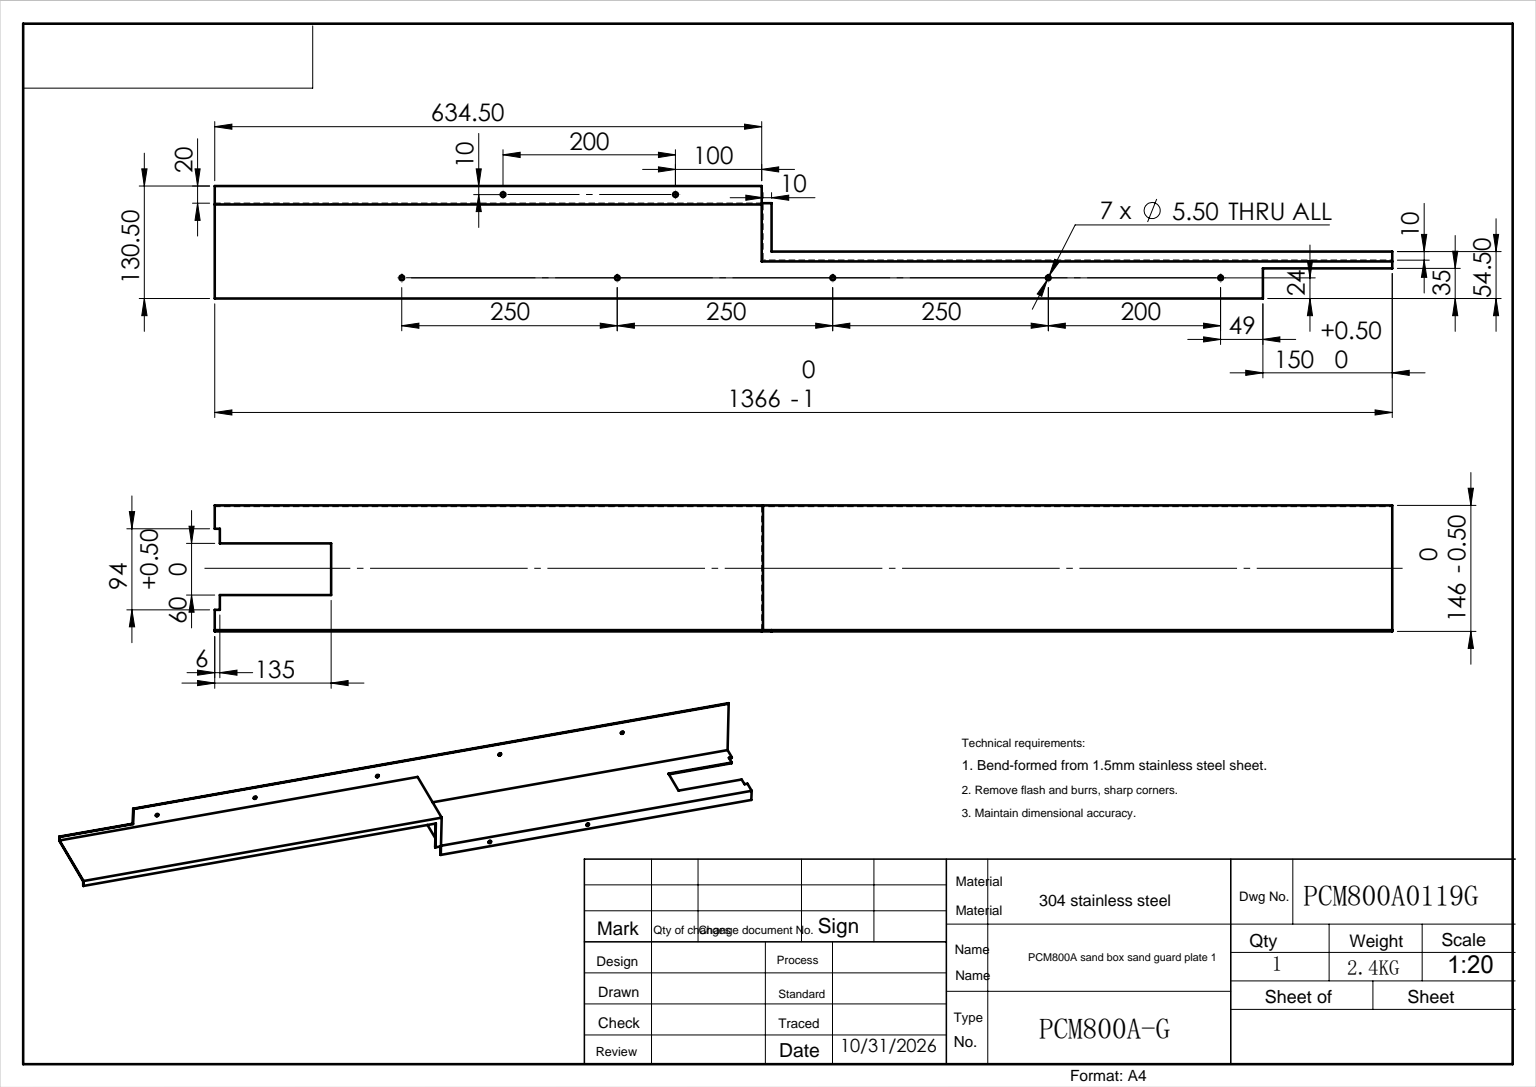
from build123d import *

# Parameters (mm, degrees)
SKETCH_1_W                  = 146
SKETCH_1_H                  = 636
EXTRUDE_1_DEPTH             = 1.5
SKETCH_2_W                  = 1.5
SKETCH_2_H                  = 636
EXTRUDE_2_DEPTH             = 109
SKETCH_4_W                  = 144.5
SKETCH_4_H                  = 1.5
EXTRUDE_4_DEPTH             = 66
EXTRUDE_5_DEPTH             = 730
SKETCH_6_W                  = 1.5
SKETCH_6_H                  = 634.5
EXTRUDE_6_DEPTH             = 20
SKETCH_7_W                  = 1.5
SKETCH_7_H                  = 730
EXTRUDE_7_DEPTH             = 10
SKETCH_8_W                  = 1.5
SKETCH_8_H                  = 56
EXTRUDE_8_DEPTH             = 10
SKETCH_10_W                 = 35
SKETCH_10_H                 = 150
CUT_EXTRUDE_2_DEPTH         = 2
HOLE_WIZARD_5_5_5_5_1_D     = 5.5
HOLE_WIZARD_5_5_5_5_2_D     = 5.5
HOLE_WIZARD_5_5_5_5_2_DEPTH = 1.5
HOLE_WIZARD_5_5_5_5_2_TIP   = 1.652366702
CUT_EXTRUDE_3_DEPTH         = 55


with BuildPart() as part:
    # 草图1 → 凸台-拉伸1 (new body)
    with BuildSketch(Plane.XY):
        with Locations((73, 318)):
            Rectangle(SKETCH_1_W, SKETCH_1_H)
    extrude(amount=EXTRUDE_1_DEPTH)

    # 草图2 → 凸台-拉伸2 (add)
    with BuildSketch(Plane.XY.offset(1.5)):
        with Locations((0.75, 318)):
            Rectangle(SKETCH_2_W, SKETCH_2_H)
    extrude(amount=EXTRUDE_2_DEPTH)

    # 草图4 → 凸台-拉伸4 (add)
    with BuildSketch(Plane.XY.offset(1.5)):
        with Locations((73.75, 0.75)):
            Rectangle(SKETCH_4_W, SKETCH_4_H)
    extrude(amount=EXTRUDE_4_DEPTH)

    # 草图5 → 凸台-拉伸5 (add)
    with BuildSketch(Plane.XZ):
        Polygon((0, 110.5), (0, 66), (146, 66), (146, 67.5), (1.5, 67.5), (1.5, 110.5), align=None)
    extrude(amount=EXTRUDE_5_DEPTH)

    # 草图6 → 凸台-拉伸6 (add)
    with BuildSketch(Plane(origin=(0, 0, 0), x_dir=(-1, 0, 0), z_dir=(0, 0, -1))):
        with Locations((-145.25, 318.75)):
            Rectangle(SKETCH_6_W, SKETCH_6_H)
    extrude(amount=EXTRUDE_6_DEPTH)

    # 草图7 → 凸台-拉伸7 (add)
    with BuildSketch(Plane(origin=(0, 0, 66), x_dir=(-1, 0, 0), z_dir=(0, 0, -1))):
        with Locations((-145.25, -365)):
            Rectangle(SKETCH_7_W, SKETCH_7_H)
    extrude(amount=EXTRUDE_7_DEPTH)

    # 草图8 → 凸台-拉伸8 (add)
    with BuildSketch(Plane.XZ):
        with Locations((145.25, 28)):
            Rectangle(SKETCH_8_W, SKETCH_8_H)
    extrude(amount=EXTRUDE_8_DEPTH)

    # 草图10 → 切除-拉伸2 (cut)
    with BuildSketch(Plane(origin=(1.5, 0, 0), x_dir=(0, 0, -1), z_dir=(1, 0, 0))):
        with Locations((-93, -655)):
            Rectangle(SKETCH_10_W, SKETCH_10_H)
    extrude(amount=-CUT_EXTRUDE_2_DEPTH, mode=Mode.SUBTRACT)

    # Ø5.5 (5.5) 直径孔1 (through all)
    with Locations(Plane(origin=(1.5, 0, 0), x_dir=(0, 0, -1), z_dir=(1, 0, 0))):
        with Locations((-86.5, 419), (-86.5, 169), (-86.5, -81), (-86.5, -331), (-86.5, -531)):
            Hole(HOLE_WIZARD_5_5_5_5_1_D / 2)

    # Ø5.5 (5.5) 直径孔2
    with Locations(Plane.ZY.offset(-144.5)):
        with Locations((-10, 301.5), (-10, 101.5)):
            Hole(HOLE_WIZARD_5_5_5_5_2_D / 2, depth=HOLE_WIZARD_5_5_5_5_2_DEPTH)
            with Locations((0, 0, -(HOLE_WIZARD_5_5_5_5_2_DEPTH + HOLE_WIZARD_5_5_5_5_2_TIP / 2))):  # 118° drill point
                Cone(0, HOLE_WIZARD_5_5_5_5_2_D / 2, HOLE_WIZARD_5_5_5_5_2_TIP, mode=Mode.SUBTRACT)

    # 草图15 → 切除-拉伸3 (cut)
    with BuildSketch(Plane.XY.offset(1.5)):
        Polygon((27, 636), (27, 630), (44, 630), (44, 501), (104, 501), (104, 630), (121, 630), (121, 636), align=None)
    extrude(amount=-CUT_EXTRUDE_3_DEPTH, mode=Mode.SUBTRACT)


solid = part.part
